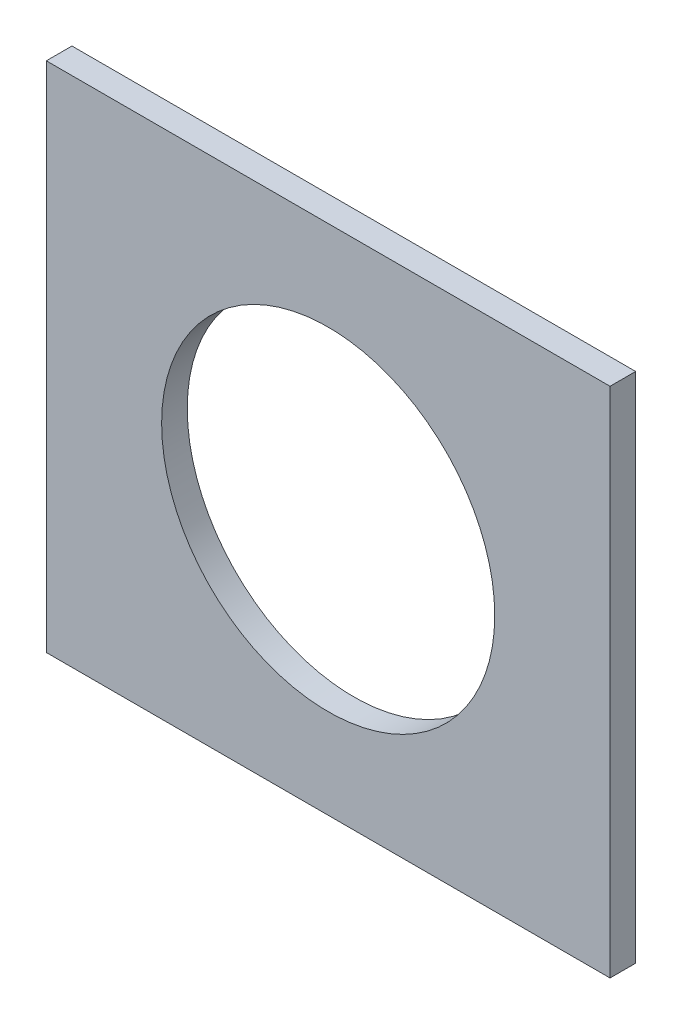
SolidWorks part; units mm, degrees
ref_plane "前视基准面" through (0, 0, 0) normal (0, 0, 1) x (1, 0, 0)
ref_plane "上视基准面" through (0, 0, 0) normal (0, 1, 0) x (1, 0, 0)
ref_plane "右视基准面" through (0, 0, 0) normal (1, 0, 0) x (0, 0, -1)
sketch "草图1" plane through (0, 0, 0) normal (0, 0, 1) x (1, 0, 0)
  line L0 (0, 0) -> (110, 0)
  line L1 (110, 0) -> (110, 100)
  line L2 (110, 100) -> (0, 100)
  line L3 (0, 100) -> (0, 0)
extrude "凸台-拉伸1" add sketch "草图1" along normal blind 5
sketch "草图2" plane through (0, 0, 5) normal (0, 0, 1) x (1, 0, 0)
  line L0 (110, 100) -> (0, 0)
  line L1 (55, 50) -> (55, 82.5)
  circle A0 centre (55, 50) radius 32.5
extrude "切除-拉伸1" cut sketch "草图2" against normal blind 5 contours L0 A0 L1 | L1 A0 L0 | L0 A0
sketch "草图3" plane through (110, 0, 0) normal (1, 0, 0) x (0, 0, -1)
  line L8 (0, 0) -> (0, 100)
  line L9 (0, 100) -> (-5, 100)
  line L10 (-5, 100) -> (-5, 0)
  line L11 (-5, 0) -> (0, 0)
  line L12 (0, 0) -> (0, 100)
  line L13 (0, 100) -> (-5, 100)
  line L14 (-5, 100) -> (-5, 0)
  line L15 (-5, 0) -> (0, 0)
  dimension "D1" = 0
extrude "凸台-拉伸2" add sketch "草图3" along normal blind 50
sketch "草图4" plane through (0, 0, 0) normal (-1, 0, 0) x (0, 0, 1)
  line L8 (0, 100) -> (0, 0)
  line L9 (0, 0) -> (5, 0)
  line L10 (5, 0) -> (5, 100)
  line L11 (5, 100) -> (0, 100)
  line L12 (0, 100) -> (0, 0)
  line L13 (0, 0) -> (5, 0)
  line L14 (5, 0) -> (5, 100)
  line L15 (5, 100) -> (0, 100)
  dimension "D1" = 0
extrude "凸台-拉伸3" add sketch "草图4" along normal blind 50
sketch "草图5" plane through (160, 0, 0) normal (1, 0, 0) x (0, 0, -1)
  line L8 (-5, 0) -> (0, 0)
  line L9 (0, 0) -> (0, 100)
  line L10 (0, 100) -> (-5, 100)
  line L11 (-5, 100) -> (-5, 0)
  line L12 (-5, 0) -> (0, 0)
  line L13 (0, 0) -> (0, 100)
  line L14 (0, 100) -> (-5, 100)
  line L15 (-5, 100) -> (-5, 0)
  dimension "D1" = 0
extrude "切除-拉伸2" cut sketch "草图5" against normal blind 50
sketch "草图7" plane through (-50, 0, 0) normal (-1, 0, 0) x (0, 0, 1)
  line L8 (5, 100) -> (0, 100)
  line L9 (0, 100) -> (0, 0)
  line L10 (0, 0) -> (5, 0)
  line L11 (5, 0) -> (5, 100)
  line L12 (5, 100) -> (0, 100)
  line L13 (0, 100) -> (0, 0)
  line L14 (0, 0) -> (5, 0)
  line L15 (5, 0) -> (5, 100)
  dimension "D1" = 0
extrude "切除-拉伸3" cut sketch "草图7" against normal blind 50
